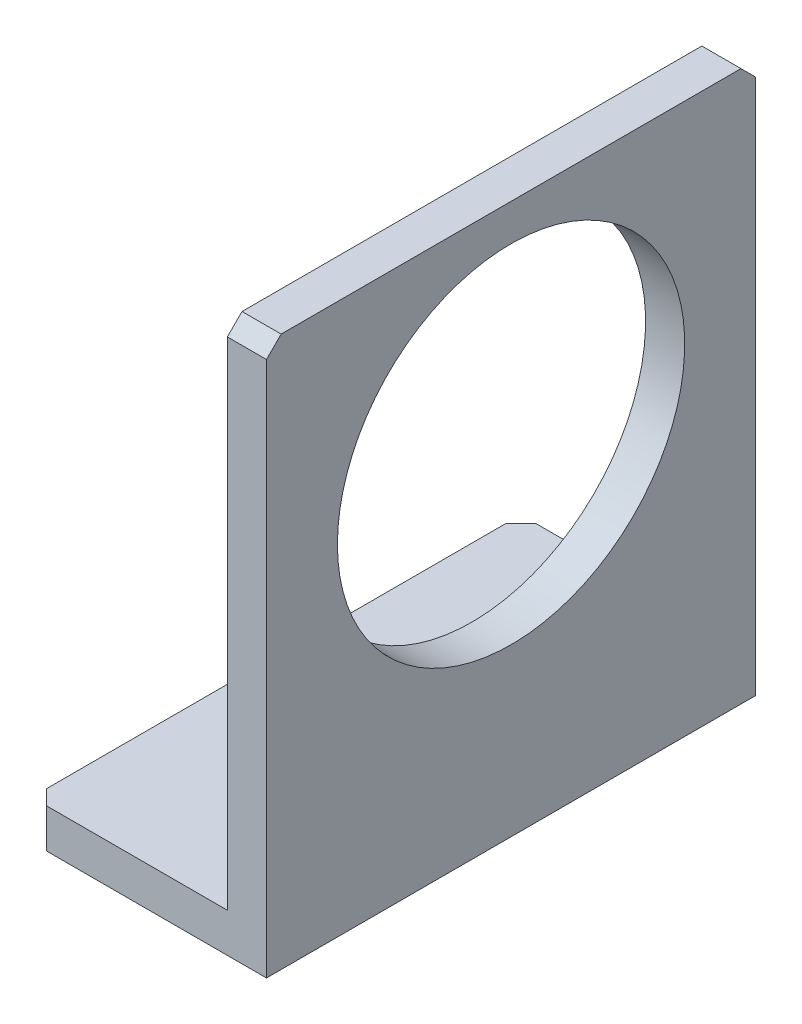
SolidWorks part; units mm, degrees
ref_plane "前视基准面" through (0, 0, 0) normal (0, 0, 1) x (1, 0, 0)
ref_plane "上视基准面" through (0, 0, 0) normal (0, 1, 0) x (1, 0, 0)
ref_plane "右视基准面" through (0, 0, 0) normal (1, 0, 0) x (0, 0, -1)
sketch "草图2" plane through (409.6376, 0.5, -34.3795) normal (0, 0, 1) x (1, 0, 0)
  line L0 (-409.6376, 112) -> (-409.6376, -0.5)
  line L1 (-409.6376, -0.5) -> (-457.6376, -0.5)
  line L2 (-457.6376, -0.5) -> (-457.6376, 7.5)
  line L3 (-457.6376, 7.5) -> (-417.6376, 7.5)
  line L4 (-417.6376, 7.5) -> (-417.6376, 112)
  line L5 (-417.6376, 112) -> (-409.6376, 112)
  dimension "D2" = 8
  dimension "D3" = 8
  dimension "D4" = 104.5
  dimension "D5" = 40
extrude "凸台-拉伸1" add sketch "草图2" along normal mid plane 100
chamfer "倒角1" distance 3 angle 45 4 edges at (-48, 4, -84.3795) (-48, 4, 15.6205) (-4, 112.5, 15.6205) (-4, 112.5, -84.3795)
sketch "草图4" plane through (-8, 0, 0) normal (-1, 0, 0) x (0, 0, 1)
  line L0 (-34.3795, 69.5) -> (-34.3795, 112.5) construction
  line L1 (12.6205, 112.5) -> (-81.3795, 112.5) construction
  circle A0 centre (-34.3795, 69.5) radius 35.5
  dimension "D2" = 71
  dimension "D1" = 43
extrude "切除-拉伸1" cut sketch "草图4" against normal up to next
